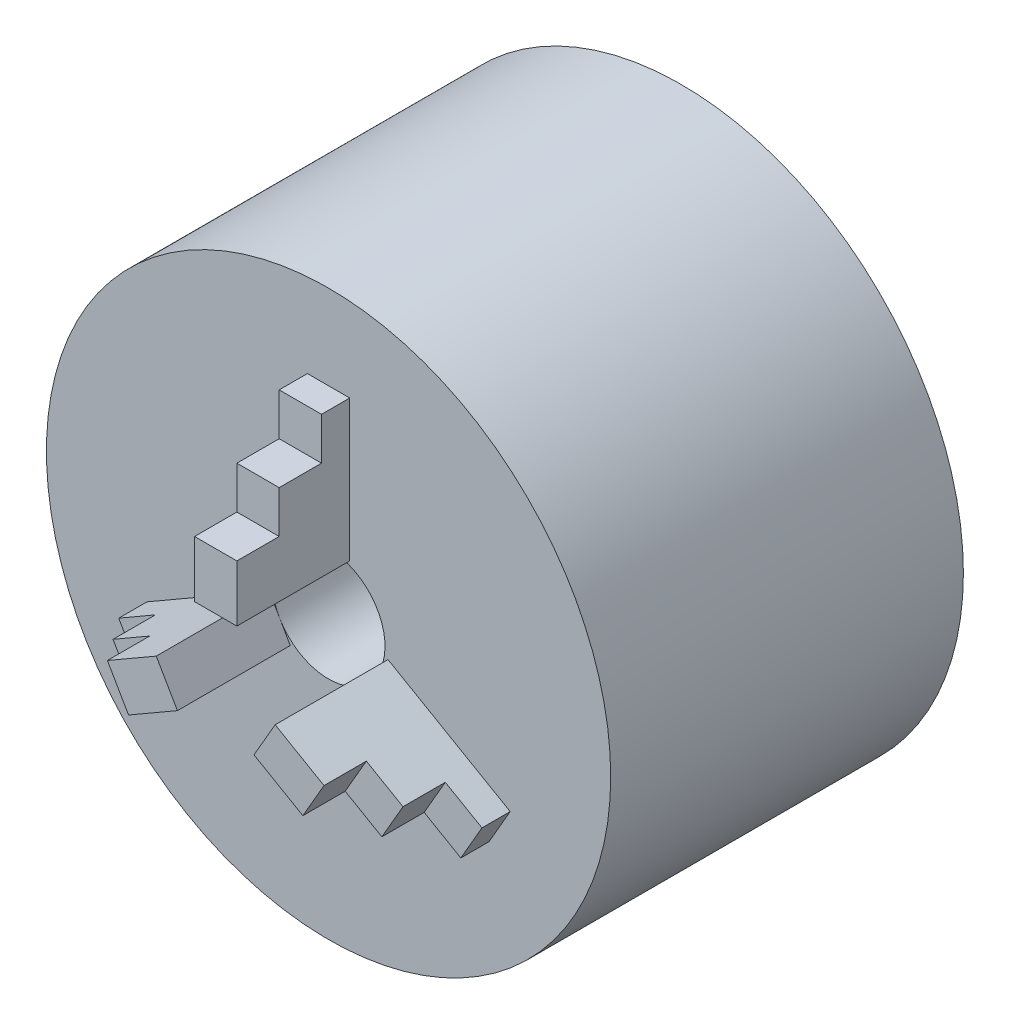
from build123d import *

# Parameters (mm, degrees)
SKETCH_1_R               = 40
EXTRUDE_1_DEPTH          = 50
SKETCH_2_W               = 6
SKETCH_2_H               = 20
EXTRUDE_2_DEPTH          = 16
CUT_EXTRUDE_1_DEPTH      = 89.345911054
PATTERN_CIRCULAR_1_COUNT = 3
SKETCH_4_R               = 8
CUT_EXTRUDE_2_DEPTH      = 87.925255248
PATTERN_CIRCULAR_2_COUNT = 3


with BuildPart() as part:
    # 草图1 → 凸台-拉伸1 (new body)
    with BuildSketch(Plane.XY):
        Circle(SKETCH_1_R)
    extrude(amount=EXTRUDE_1_DEPTH)

    # 草图2 → 凸台-拉伸2 (add)
    with BuildSketch(Plane.XY.offset(50)):
        with Locations((0, 18)):
            Rectangle(SKETCH_2_W, SKETCH_2_H)
    extrude_2 = extrude(amount=EXTRUDE_2_DEPTH)

    # 草图3 → 切除-拉伸1 (cut, through all)
    with BuildSketch(Plane.ZY.offset(3)):
        Polygon((54, 28), (54, 22), (60, 22), (60, 16), (66, 16), (66, 28), align=None)
    cut_extrude_1 = extrude(amount=-CUT_EXTRUDE_1_DEPTH, mode=Mode.SUBTRACT)

    # 阵列(圆周)1: 凸台-拉伸2, 切除-拉伸1 ×3 about axis
    pattern_circular_1_axis = Axis((0, 0, 0), (0, 0, 1))
    add([extrude_2.rotate(pattern_circular_1_axis, i * 360 / PATTERN_CIRCULAR_1_COUNT) for i in range(1, PATTERN_CIRCULAR_1_COUNT)])
    add([cut_extrude_1.rotate(pattern_circular_1_axis, i * 360 / PATTERN_CIRCULAR_1_COUNT) for i in range(1, PATTERN_CIRCULAR_1_COUNT)], mode=Mode.SUBTRACT)

    # 草图4 → 切除-拉伸2 (cut, through all)
    with BuildSketch(Plane(origin=(0, 0, 0), x_dir=(-1, 0, 0), z_dir=(0, 0, -1))):
        Circle(SKETCH_4_R)
    extrude(amount=-CUT_EXTRUDE_2_DEPTH, mode=Mode.SUBTRACT)

    # 草图5 → M6 螺纹孔1 (revolve, cut)
    with BuildSketch(Plane(origin=(0, 33, 0), x_dir=(0, 1, 0), z_dir=(1, 0, 0))):
        Polygon((0, 0), (0, 18.502151548), (2.5, 17), (2.5, 0), align=None)
    hole_wizard_m6_1 = revolve(axis=Axis((0, 33, -6.35), (0, 0, 1)), mode=Mode.SUBTRACT)

    # 阵列(圆周)2: M6 螺纹孔1 ×3 about axis
    pattern_circular_2_axis = Axis((0, 0, 0), (0, 0, 1))
    for i in range(1, PATTERN_CIRCULAR_2_COUNT):
        add(hole_wizard_m6_1.rotate(pattern_circular_2_axis, i * 360 / PATTERN_CIRCULAR_2_COUNT), mode=Mode.SUBTRACT)


solid = part.part
